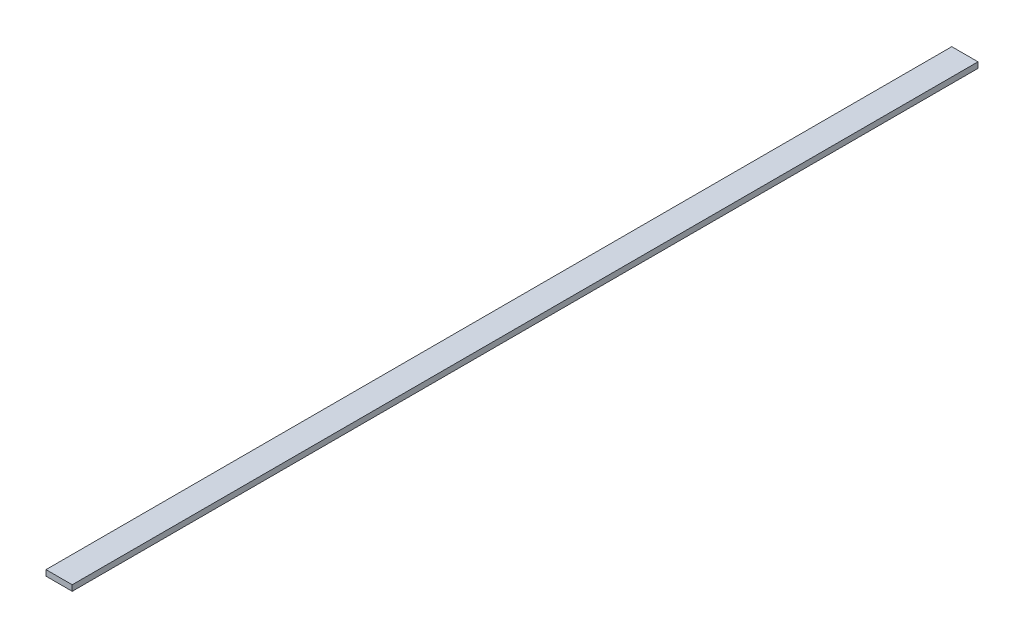
from build123d import *

# Parameters (mm, degrees)
SKETCH_1_W      = 55
SKETCH_1_H      = 12
EXTRUDE_1_DEPTH = 1900


with BuildPart() as part:
    # 草图1 → 凸台-拉伸1 (new body)
    with BuildSketch(Plane.XY):
        with Locations((27.5, -6)):
            Rectangle(SKETCH_1_W, SKETCH_1_H)
    extrude(amount=EXTRUDE_1_DEPTH)


solid = part.part
